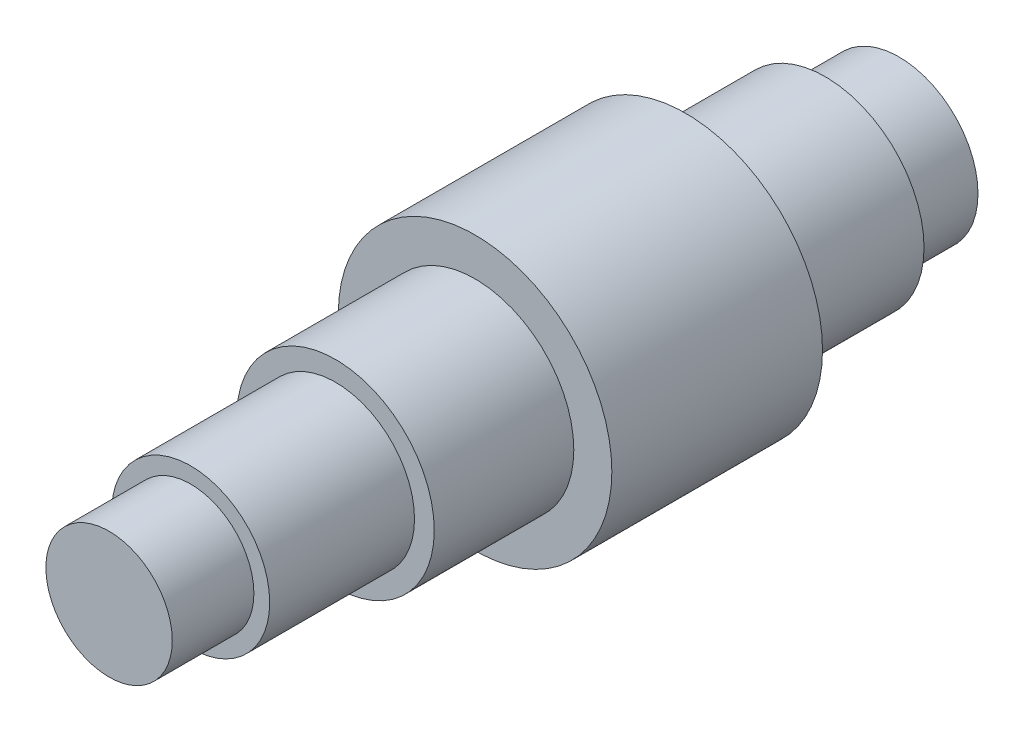
SolidWorks part; units mm, degrees
ref_plane "Front Plane" through (0, 0, 0) normal (0, 0, 1) x (1, 0, 0)
ref_plane "Top Plane" through (0, 0, 0) normal (0, 1, 0) x (1, 0, 0)
ref_plane "Right Plane" through (0, 0, 0) normal (1, 0, 0) x (0, 0, -1)
sketch "Sketch1" plane through (0, 0, 0) normal (0, 0, 1) x (1, 0, 0)
  circle A0 centre (0, 0) radius 30
  dimension "D1" = 60
extrude "Boss-Extrude1" add sketch "Sketch1" along normal blind 28
sketch "Sketch2" plane through (0, 0, 28) normal (0, 0, 1) x (1, 0, 0)
  circle A0 centre (0, 0) radius 37.5
  dimension "D1" = 75
extrude "Boss-Extrude2" add sketch "Sketch2" along normal blind 53
sketch "Sketch3" plane through (0, 0, 81) normal (0, 0, 1) x (1, 0, 0)
  circle A0 centre (0, 0) radius 51.9465
  dimension "D1" = 103.893
extrude "Boss-Extrude3" add sketch "Sketch3" along normal blind 80
sketch "Sketch4" plane through (0, 0, 161) normal (0, 0, 1) x (1, 0, 0)
  circle A0 centre (0, 0) radius 37.5
  dimension "D1" = 75
extrude "Boss-Extrude4" add sketch "Sketch4" along normal blind 53
sketch "Sketch5" plane through (0, 0, 214) normal (0, 0, 1) x (1, 0, 0)
  circle A0 centre (0, 0) radius 30
  dimension "D1" = 60
extrude "Boss-Extrude5" add sketch "Sketch5" along normal blind 55
sketch "Sketch6" plane through (0, 0, 269) normal (0, 0, 1) x (1, 0, 0)
  circle A0 centre (0, 0) radius 24
  dimension "D1" = 48
extrude "Boss-Extrude6" add sketch "Sketch6" along normal blind 31
